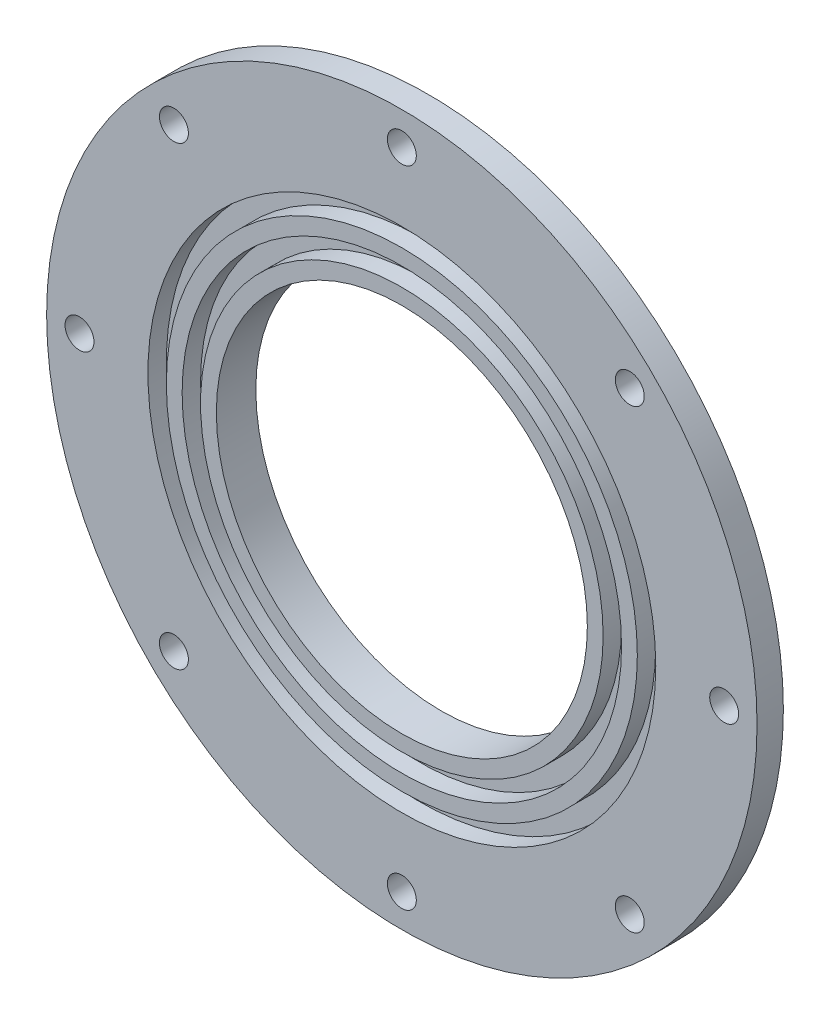
from build123d import *

# Parameters (mm, degrees)
SKETCH2_R          = 11
CUT_EXTRUDE1_DEPTH = 41
CIRPATTERN1_COUNT  = 8


with BuildPart() as part:
    # Sketch1 → Revolve1 (revolve)
    with BuildSketch(Plane(origin=(0, 0, 0), x_dir=(0, 0, -1), z_dir=(1, 0, 0)), mode=Mode.PRIVATE) as revolve1_sk:
        Polygon((0, 141), (0, 153), (14, 153), (14, 167), (0, 167), (0, 179), (14, 179), (14, 193), (0, 193), (0, 270), (20, 270), (20, 220), (45, 220), (45, 200), (30, 200), (30, 141), align=None)
    revolve(revolve1_sk.sketch.rotate(Axis((0, 0, 0), (0, 0, -1)), 90), axis=Axis((0, 0, 0), (0, 0, -1)))

    # Sketch2 → Cut-Extrude1 (cut)
    with BuildSketch(Plane.XY):
        with Locations((0, 245)):
            Circle(SKETCH2_R)
    cut_extrude1 = extrude(amount=-CUT_EXTRUDE1_DEPTH, mode=Mode.SUBTRACT)

    # CirPattern1: Cut-Extrude1 ×8 about axis
    cirpattern1_axis = Axis((0, 0, 0), (0, 0, 1))
    for i in range(1, CIRPATTERN1_COUNT):
        add(cut_extrude1.rotate(cirpattern1_axis, i * 360 / CIRPATTERN1_COUNT), mode=Mode.SUBTRACT)


solid = part.part
